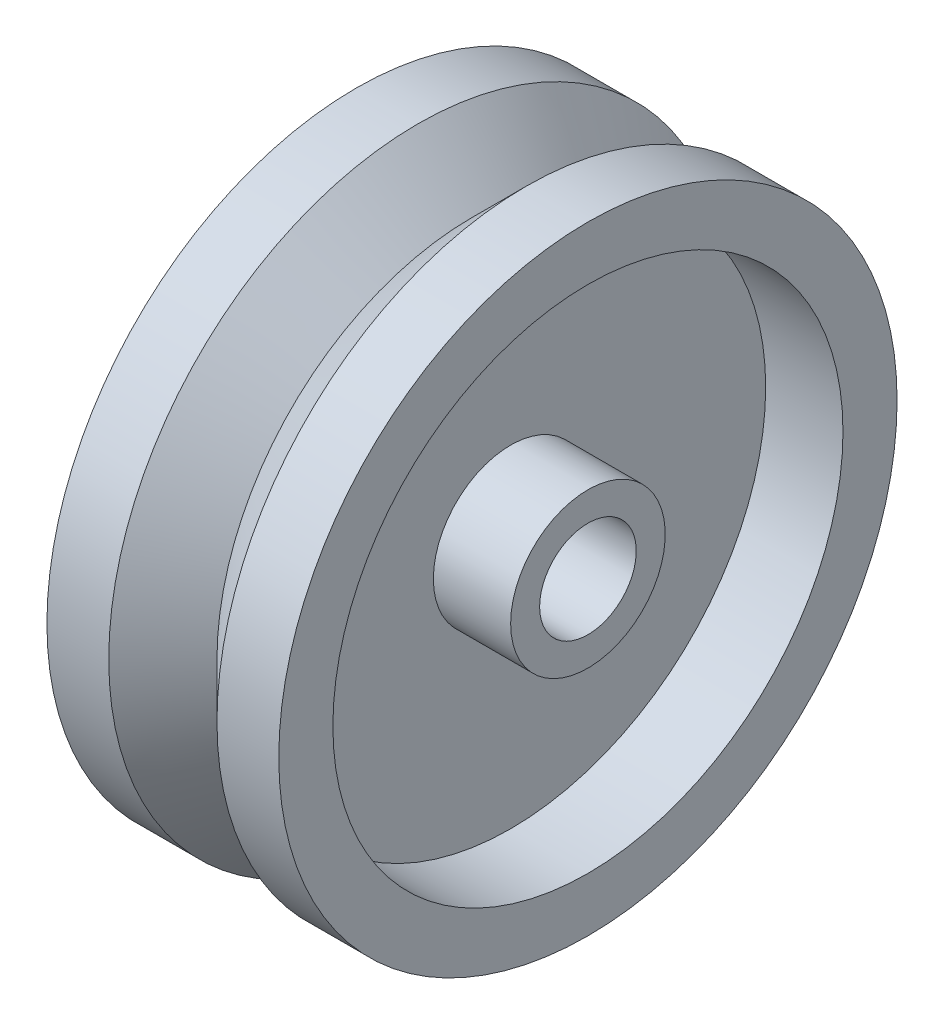
from build123d import *


with BuildPart() as part:
    # Sketch1 → Revolve1 (revolve)
    with BuildSketch(Plane.XY, mode=Mode.PRIVATE) as revolve1_sk:
        Polygon((3.5, 20), (0, 16.5), (-3.5, 20), (-7.5, 20), (-7.5, 16.5), (-2.5, 16.5), (-2.5, 5), (-7.5, 5), (-7.5, 3.125), (7.5, 3.125), (7.5, 5), (2.5, 5), (2.5, 16.5), (7.5, 16.5), (7.5, 20), align=None)
    revolve(revolve1_sk.sketch.rotate(Axis((-45.5, 0, 0), (1, 0, 0)), 90), axis=Axis((-45.5, 0, 0), (1, 0, 0)))


solid = part.part
